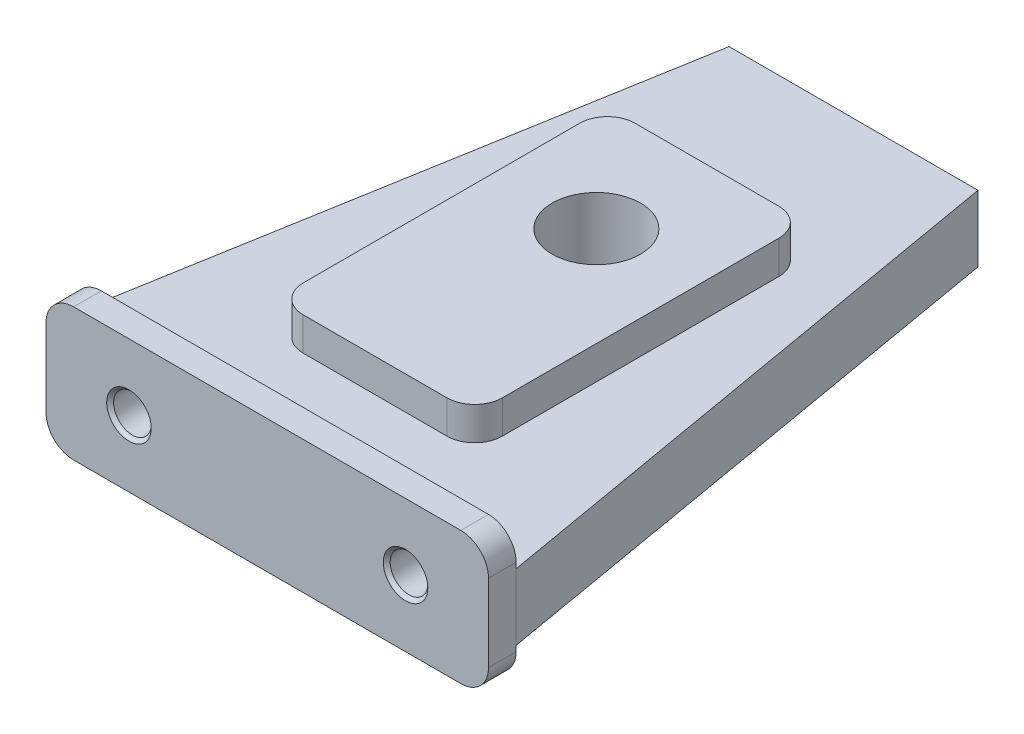
SolidWorks part; units mm, degrees
ref_plane "Front Plane" through (0, 0, 0) normal (0, 0, 1) x (1, 0, 0)
ref_plane "Top Plane" through (0, 0, 0) normal (0, 1, 0) x (1, 0, 0)
ref_plane "Right Plane" through (0, 0, 0) normal (1, 0, 0) x (0, 0, -1)
sketch "Sketch1" plane through (0, 0, 0) normal (0, 0, 1) x (1, 0, 0)
  line L1 (-35, -12) -> (35, -12)
  line L2 (-40, -7) -> (-40, 7)
  line L3 (-35, 12) -> (35, 12)
  line L4 (40, -7) -> (40, 7)
  line L5 (-40, -12) -> (40, 12) construction
  line L6 (-40, 12) -> (40, -12) construction
  arc A0 (35, 12) -> (40, 7) centre (35, 7) cw
  arc A1 (35, -12) -> (40, -7) centre (35, -7) ccw
  arc A2 (-35, -12) -> (-40, -7) centre (-35, -7) cw
  arc A3 (-40, 7) -> (-35, 12) centre (-35, 7) cw
  point P0 (0, 0)
  dimension "D3" = 5
  dimension "D1" = 80
  dimension "D2" = 24
extrude "Boss-Extrude1" add sketch "Sketch1" along normal blind 5
sketch "Sketch2" plane through (0, 0, 0) normal (0, 1, 0) x (1, 0, 0)
  line L0 (-40, 0) -> (-22.5, 101)
  line L1 (-22.5, 101) -> (22.5, 101)
  line L2 (22.5, 101) -> (40, 0)
  line L3 (40, 0) -> (-40, 0)
  line L4 (35, -5) -> (-35, -5) construction
  point P3 (0, 101)
  dimension "D1" = 45
  dimension "D2" = 106
extrude "Boss-Extrude2" add sketch "Sketch2" along normal mid plane 12
sketch "Sketch3" plane through (0, 6, 0) normal (0, 1, 0) x (1, 0, 0)
  line L0 (22.5, 101) -> (-22.5, 101) construction
  line L1 (-13, 14.5) -> (13, 14.5)
  line L2 (-18, 19.5) -> (-18, 69.5)
  line L3 (-13, 74.5) -> (13, 74.5)
  line L4 (18, 19.5) -> (18, 69.5)
  line L5 (-18, 14.5) -> (18, 74.5) construction
  line L6 (-18, 74.5) -> (18, 14.5) construction
  arc A0 (-13, 14.5) -> (-18, 19.5) centre (-13, 19.5) cw
  arc A1 (13, 14.5) -> (18, 19.5) centre (13, 19.5) ccw
  arc A2 (-18, 69.5) -> (-13, 74.5) centre (-13, 69.5) cw
  arc A3 (13, 74.5) -> (18, 69.5) centre (13, 69.5) cw
  point P0 (0, 44.5)
  dimension "D4" = 5
  dimension "D1" = 26.5
  dimension "D2" = 60
  dimension "D3" = 36
extrude "Boss-Extrude3" add sketch "Sketch3" along normal blind 6
sketch "Sketch4" plane through (0, 12, 0) normal (0, 1, 0) x (1, 0, 0)
  line L0 (22.5, 101) -> (-22.5, 101) construction
  circle A0 centre (0, 54.5) radius 8
  dimension "D1" = 16
  dimension "D2" = 46.5
extrude "Cut-Extrude1" cut sketch "Sketch4" against normal blind 21
sketch "Sketch5" plane through (0, 0, 5) normal (0, 0, 1) x (1, 0, 0)
  point P0 (-25, 0)
  point P1 (25, 0)
  dimension "D1" = 25
  dimension "D2" = 25
sketch "Sketch6" plane through (0, 0, -101) normal (0, 0, -1) x (-1, 0, 0)
  point P0 (-14, 0)
  point P1 (14, 0)
  dimension "D1" = 14
  dimension "D2" = 14
hole_wizard "M8 Tapped Hole1" positions "3DSketch1" profile "Sketch7" tap size "M8" standard "GB"
sketch3d "3DSketch1"
  point P0 (25, 0, 5)
  point P3 (-25, 0, 5)
sketch "Sketch7" plane through (25, 0, 5) normal (1, 0, 0) x (0, -1, 0)
  line L0 (0, 0) -> (0, 22.0429)
  line L1 (0, 22.0429) -> (3.4, 20)
  line L2 (3.4, 20) -> (3.4, 0.625)
  line L3 (3.4, 0.625) -> (4.025, 0)
  line L5 (4.025, 0) -> (0, 0)
  line L6 (-3.4, 0.625) -> (-4.025, 0) construction
  line L10 (0, 22.0429) -> (-3.4, 20) construction
  line L11 (0, -6.35) -> (0, 107.95) construction
  dimension "螺纹孔钻头直径" = 6.8
  dimension "螺纹孔钻头深度" = 20
  dimension "近端锥形沉头孔直径" = 8.05
  dimension "近端锥形沉头孔角度" = 90
  dimension "导头角度" = 118
cosmetic thread "Hole Thread1"
cosmetic thread "Hole Thread2"
hole_wizard "M6 Tapped Hole1" positions "3DSketch2" profile "Sketch8" tap size "M6" standard "GB"
sketch3d "3DSketch2"
  point P0 (14, 0, -101)
  point P3 (-14, 0, -101)
sketch "Sketch8" plane through (14, 0, -101) normal (1, 0, 0) x (0, 1, 0)
  line L0 (0, 0) -> (0, 11.5022)
  line L1 (0, 11.5022) -> (2.5, 10)
  line L2 (2.5, 10) -> (2.5, 0.525)
  line L3 (2.5, 0.525) -> (3.025, 0)
  line L5 (3.025, 0) -> (0, 0)
  line L6 (-2.5, 0.525) -> (-3.025, 0) construction
  line L10 (0, 11.5022) -> (-2.5, 10) construction
  line L11 (0, -6.35) -> (0, 107.95) construction
  dimension "螺纹孔钻头直径" = 5
  dimension "螺纹孔钻头深度" = 10
  dimension "近端锥形沉头孔直径" = 6.05
  dimension "近端锥形沉头孔角度" = 90
  dimension "导头角度" = 118
cosmetic thread "Hole Thread3" parameters "D1"=12, "D2"=6
cosmetic thread "Hole Thread4" parameters "D1"=12, "D2"=6
